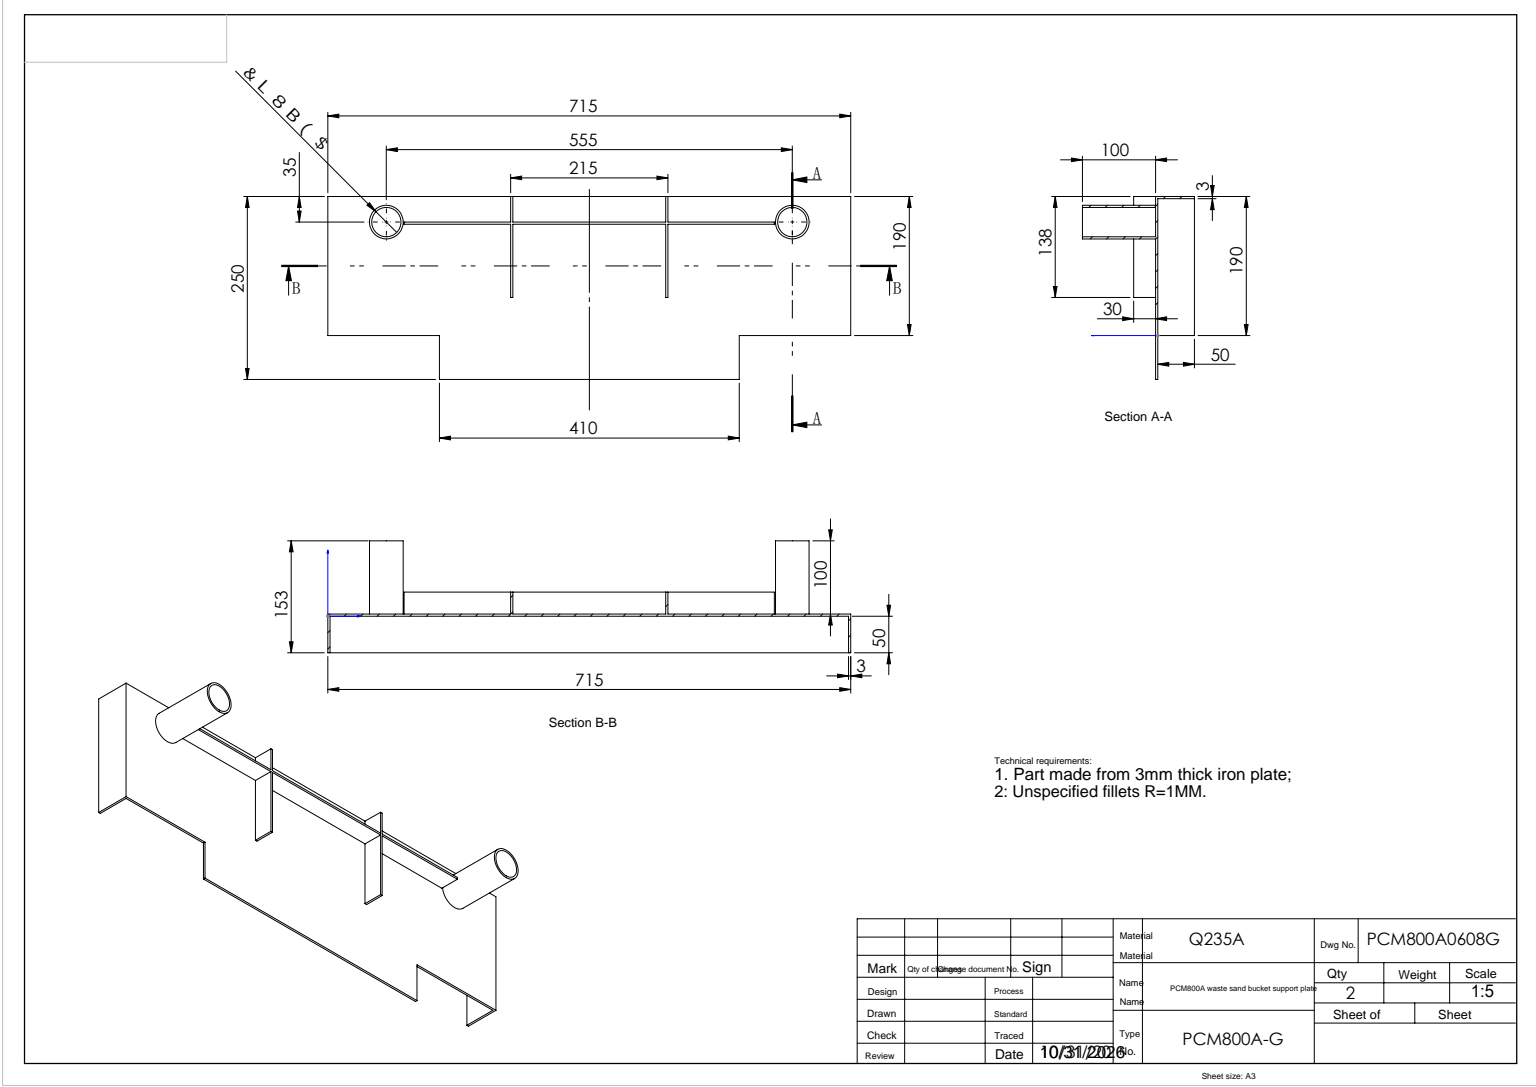
from build123d import *

# Parameters (mm, degrees)
EXTRUDE_1_DEPTH  = 3
SKETCH_2_R       = 23
SKETCH_2_R_2     = 20
EXTRUDE_2_DEPTH  = 100
SKETCH_4_W       = 3
SKETCH_4_H       = 50
EXTRUDE_3_DEPTH  = 715
SKETCH_7_W       = 506.314990664
SKETCH_7_H       = 3
EXTRUDE_8_DEPTH  = 30
SKETCH_8_W       = 3
SKETCH_8_H       = 35
SKETCH_8_H_2     = 100
EXTRUDE_9_DEPTH  = 30
SKETCH_9_W       = 3
SKETCH_9_H       = 50
EXTRUDE_10_DEPTH = 187


with BuildPart() as part:
    # 草图1 → 凸台-拉伸1 (new body)
    with BuildSketch(Plane(origin=(0, 0, 0), x_dir=(1, 0, 0), z_dir=(0, 1, 0))):
        Polygon((357.5, -60), (152.5, -60), (152.5, 0), (0, 0), (0, 190), (715, 190), (715, 0), (562.5, 0), (562.5, -60), align=None)
    extrude(amount=EXTRUDE_1_DEPTH)

    # 草图2 → 凸台-拉伸2 (add)
    # profile 1 of 2: a face of its own
    with BuildSketch(Plane(origin=(0, 3, 0), x_dir=(1, 0, 0), z_dir=(0, 1, 0))):
        with Locations(Location((80, 155, 0), (0, 0, 90))):
            Circle(SKETCH_2_R)
        with Locations(Location((80, 155, 0), (0, 0, 270))):
            Circle(SKETCH_2_R_2, mode=Mode.SUBTRACT)
    # profile 2 of 2: a face of its own
    with BuildSketch(Plane(origin=(0, 3, 0), x_dir=(1, 0, 0), z_dir=(0, 1, 0))):
        with Locations(Location((635, 155, 0), (0, 0, 90))):
            Circle(SKETCH_2_R)
        with Locations(Location((635, 155, 0), (0, 0, 270))):
            Circle(SKETCH_2_R_2, mode=Mode.SUBTRACT)
    extrude(amount=EXTRUDE_2_DEPTH)

    # 草图7 → 凸台-拉伸8 (add)
    with BuildSketch(Plane(origin=(0, 3, 0), x_dir=(1, 0, 0), z_dir=(0, 1, 0))):
        with Locations((357.381396842, 153.5)):
            Rectangle(SKETCH_7_W, SKETCH_7_H)
    extrude(amount=EXTRUDE_8_DEPTH)

    # 草图8 → 凸台-拉伸9 (add)
    with BuildSketch(Plane(origin=(0, 3, 0), x_dir=(1, 0, 0), z_dir=(0, 1, 0))):
        with Locations((251.5, 172.5)):
            Rectangle(SKETCH_8_W, SKETCH_8_H)
        with Locations((251.5, 102)):
            Rectangle(SKETCH_8_W, SKETCH_8_H_2)
        with Locations((463.5, 102)):
            Rectangle(SKETCH_8_W, SKETCH_8_H_2)
        with Locations((463.5, 172.5)):
            Rectangle(SKETCH_8_W, SKETCH_8_H)
    extrude(amount=EXTRUDE_9_DEPTH)



with BuildPart() as body_2:
    # 草图4 → 凸台-拉伸3 (new body)
    with BuildSketch(Plane(origin=(715, 0, 0), x_dir=(0, 0, -1), z_dir=(1, 0, 0))):
        with Locations((188.5, -25)):
            Rectangle(SKETCH_4_W, SKETCH_4_H)
    extrude(amount=-EXTRUDE_3_DEPTH)


with BuildPart() as part_1:
    add(part.part)

    add(body_2.part)  # 凸台-拉伸10 merges body 2
    # 草图9 → 凸台-拉伸10 (add)
    with BuildSketch(Plane.XY):
        with Locations((713.5, -25)):
            Rectangle(SKETCH_9_W, SKETCH_9_H)
        with Locations((1.5, -25)):
            Rectangle(SKETCH_9_W, SKETCH_9_H)
    extrude(amount=-EXTRUDE_10_DEPTH)


solid = part_1.part
